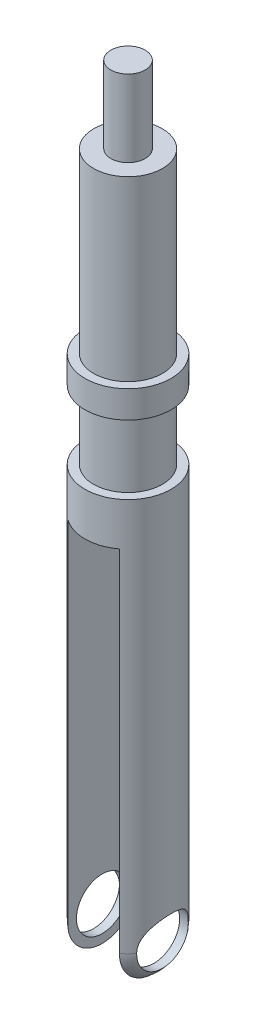
from build123d import *

# Parameters (mm, degrees)
SKETCH2_W               = 6
SKETCH2_H               = 15
CUT_EXTRUDE1_DEPTH      = 45.71
CUT_EXTRUDE2_DEPTH      = 57.171431365
CUT_EXTRUDE2_DEPTH_BACK = 19
SKETCH4_R               = 3


with BuildPart() as part:
    # Model → Revolve1 (revolve)
    with BuildSketch(Plane.XY, mode=Mode.PRIVATE) as revolve1_sk:
        with BuildLine():
            Line((-27.291095715, -5.663546948), (-27.291095715, -10.663546948))
            Line((-27.291095715, -10.663546948), (-27.291095715, -51.373546948))
            ThreePointArc((-27.291095715, -51.373546948), (-28.755561809, -54.909080854), (-32.291095715, -56.373546948))
            Line((-32.291095715, -56.373546948), (-32.291095715, -52.264917369))
            Line((-32.291095715, -52.264917369), (-32.291095715, -10.663546948))
            Line((-32.291095715, -10.663546948), (-32.291095715, 35.040839423))
            Line((-32.291095715, 35.040839423), (-30.291095715, 35.040839423))
            Line((-30.291095715, 35.040839423), (-30.291095715, 26.12431753))
            Line((-30.291095715, 26.12431753), (-28.291095715, 26.12431753))
            Line((-28.291095715, 26.12431753), (-28.291095715, 5.494079969))
            Line((-28.291095715, 5.494079969), (-27.291095715, 5.494079969))
            Line((-27.291095715, 5.494079969), (-27.291095715, 2.336453052))
            Line((-27.291095715, 2.336453052), (-28.291095714, 2.336453052))
            Line((-28.291095714, 2.336453052), (-28.291095714, -5.663546948))
            Line((-28.291095714, -5.663546948), (-27.291095715, -5.663546948))
        make_face()
    revolve(revolve1_sk.sketch.rotate(Axis((-32.291095715, 35.040839423, 0), (0, 1, 0)), 90), axis=Axis((-32.291095715, 35.040839423, 0), (0, 1, 0)))

    # Sketch2 → Cut-Extrude1 (cut)
    with BuildSketch(Plane(origin=(0, -56.373546948, 0), x_dir=(-1, 0, 0), z_dir=(0, -1, 0))):
        with Locations((32.291095715, 1.617056414)):
            Rectangle(SKETCH2_W, SKETCH2_H)
    extrude(amount=-CUT_EXTRUDE1_DEPTH, mode=Mode.SUBTRACT)

    # Sketch4 → Cut-Extrude2 (cut, two sides: drawn at the far end of the back side and taken through both)
    with BuildSketch(Plane(origin=(-35.291095715, 0, 0), x_dir=(0, 0, -1), z_dir=(1, 0, 0)).offset(-CUT_EXTRUDE2_DEPTH_BACK)):
        with Locations(Location((0, -51.373546948, 0), (0, 0, 180))):
            Circle(SKETCH4_R)
    extrude(amount=CUT_EXTRUDE2_DEPTH + CUT_EXTRUDE2_DEPTH_BACK, mode=Mode.SUBTRACT)


solid = part.part
